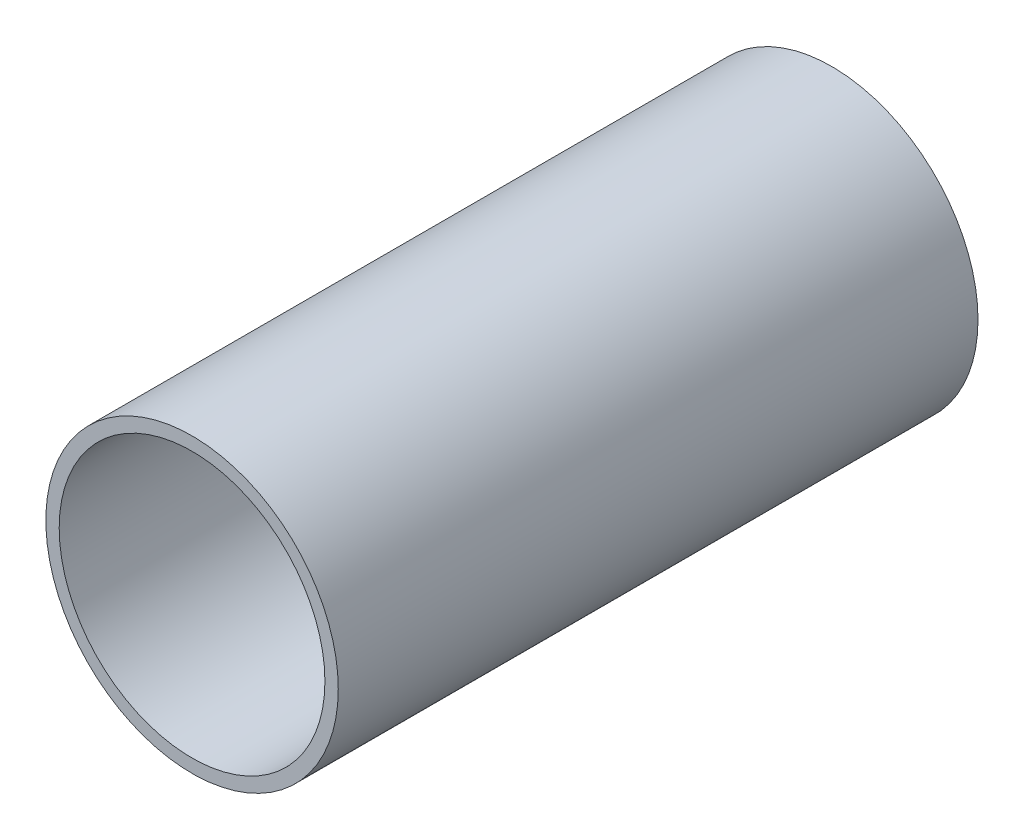
from build123d import *

# Parameters (mm, degrees)
SKETCH1_R           = 28.5
SKETCH1_R_2         = 25.9
EXTRUDE_THIN1_DEPTH = 124.7


with BuildPart() as part:
    # Sketch1 → Extrude-Thin1 (new body)
    with BuildSketch(Plane.XY):
        Circle(SKETCH1_R)
        Circle(SKETCH1_R_2, mode=Mode.SUBTRACT)
    extrude(amount=EXTRUDE_THIN1_DEPTH)


solid = part.part
